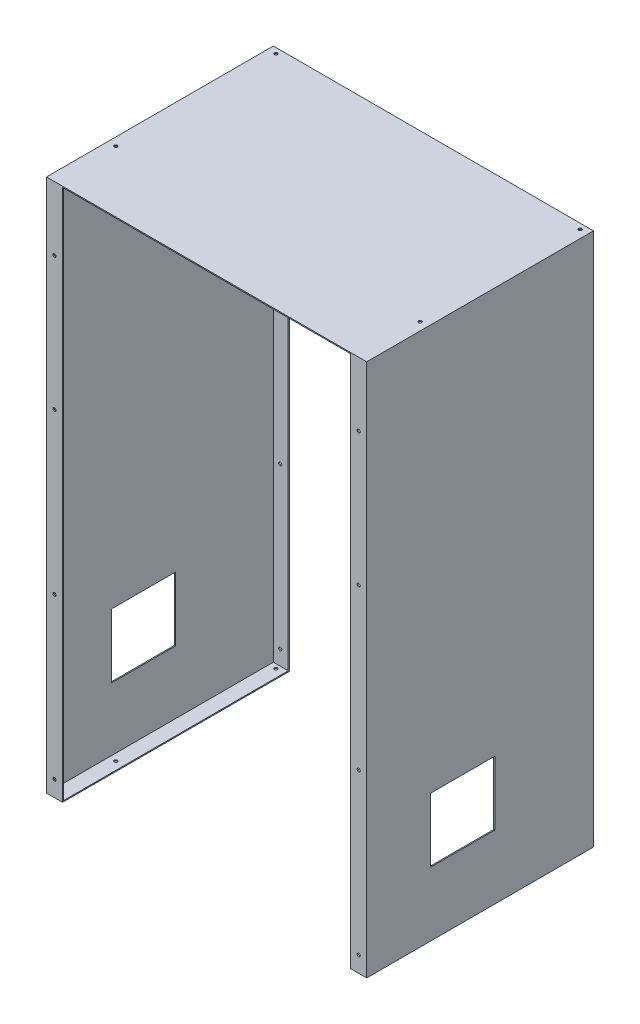
from build123d import *

# Parameters (mm, degrees)
SKETCH_1_W          = 600
SKETCH_1_H          = 425
EXTRUDE_1_DEPTH     = 1000
SHELL_2_T           = -2
SKETCH_2_W          = 540
SKETCH_2_H          = 998
CUT_EXTRUDE_1_DEPTH = 900
SKETCH_5_W          = 28
SKETCH_5_H          = 421
EXTRUDE_2_DEPTH     = 2
SKETCH_6_W          = 120
SKETCH_6_H          = 120
CUT_EXTRUDE_3_DEPTH = 812
SKETCH_7_R          = 3
CUT_EXTRUDE_4_DEPTH = 1118
SKETCH_8_R          = 3
CUT_EXTRUDE_5_DEPTH = 671


with BuildPart() as part:
    # 草图1 → 凸台-拉伸1 (new body)
    with BuildSketch(Plane(origin=(0, 0, 0), x_dir=(1, 0, 0), z_dir=(0, 1, 0))):
        with Locations((300, 212.5)):
            Rectangle(SKETCH_1_W, SKETCH_1_H)
    extrude(amount=EXTRUDE_1_DEPTH)

    # 抽壳2
    shell_2_openings = [part.faces().sort_by_distance(p)[0] for p in [
        (300, 0, -212.5),
    ]]
    offset(amount=SHELL_2_T, openings=shell_2_openings, kind=Kind.INTERSECTION)

    # 草图2 → 切除-拉伸1 (cut)
    with BuildSketch(Plane.XY):
        with Locations((300, 499)):
            Rectangle(SKETCH_2_W, SKETCH_2_H)
    extrude(amount=-CUT_EXTRUDE_1_DEPTH, mode=Mode.SUBTRACT)

    # 草图5 → 凸台-拉伸2 (add)
    with BuildSketch(Plane.XZ):
        with Locations((16, -212.5)):
            Rectangle(SKETCH_5_W, SKETCH_5_H)
        with Locations((584, -212.5)):
            Rectangle(SKETCH_5_W, SKETCH_5_H)
    extrude(amount=-EXTRUDE_2_DEPTH)

    # 草图6 → 切除-拉伸3 (cut)
    with BuildSketch(Plane(origin=(600, 0, 0), x_dir=(0, 0, -1), z_dir=(1, 0, 0))):
        with Locations((180, 180)):
            Rectangle(SKETCH_6_W, SKETCH_6_H)
    extrude(amount=-CUT_EXTRUDE_3_DEPTH, mode=Mode.SUBTRACT)

    # 草图7 → 切除-拉伸4 (cut)
    with BuildSketch(Plane.XZ):
        with Locations(Location((15, -115, 0), (0, 0, 270))):
            Circle(SKETCH_7_R)
        with Locations(Location((585, -415, 0), (0, 0, 90))):
            Circle(SKETCH_7_R)
        with Locations(Location((15, -415, 0), (0, 0, 270))):
            Circle(SKETCH_7_R)
        with Locations(Location((585, -115, 0), (0, 0, 90))):
            Circle(SKETCH_7_R)
    extrude(amount=-CUT_EXTRUDE_4_DEPTH, mode=Mode.SUBTRACT)

    # 草图8 → 切除-拉伸5 (cut)
    with BuildSketch(Plane(origin=(0, 0, -425), x_dir=(-1, 0, 0), z_dir=(0, 0, -1))):
        with Locations((-15, 30)):
            Circle(SKETCH_8_R)
        with Locations((-15, 330)):
            Circle(SKETCH_8_R)
        with Locations((-15, 630)):
            Circle(SKETCH_8_R)
        with Locations(Location((-585, 30, 0), (0, 0, 180))):
            Circle(SKETCH_8_R)
        with Locations(Location((-585, 330, 0), (0, 0, 180))):
            Circle(SKETCH_8_R)
        with Locations((-15, 880)):
            Circle(SKETCH_8_R)
        with Locations(Location((-585, 630, 0), (0, 0, 180))):
            Circle(SKETCH_8_R)
        with Locations(Location((-585, 880, 0), (0, 0, 180))):
            Circle(SKETCH_8_R)
    extrude(amount=-CUT_EXTRUDE_5_DEPTH, mode=Mode.SUBTRACT)


solid = part.part
